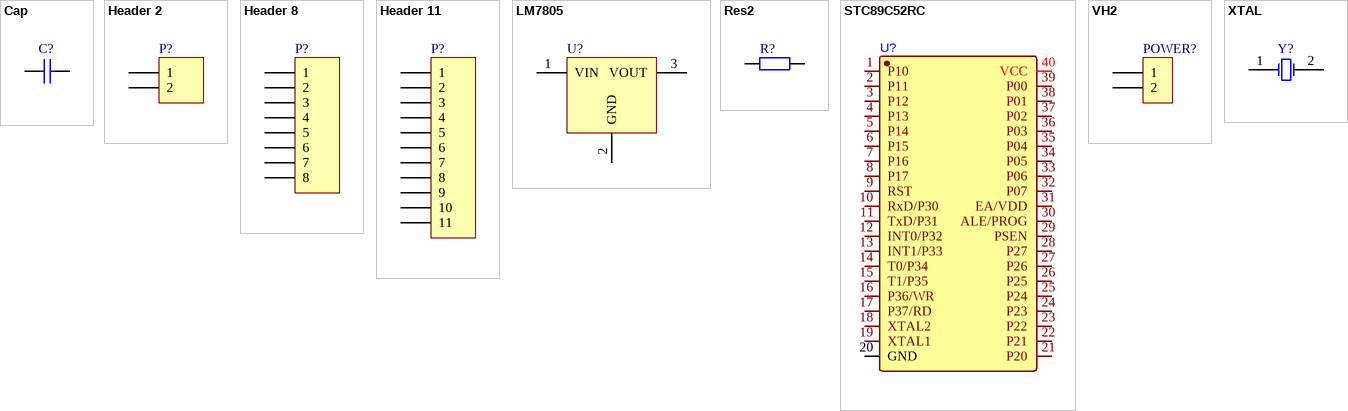
[diagram p0: symbols Cap to XTAL]
# Altium schematic symbol library MISC80679-3.SCHLIB: 9 symbols
Pins are listed as number, name and electrical type; pins without a type are passive.


## Cap
designator C?
Capacitor
simulation model CAP (Capacitor)
signal-integrity model Cap
footprint CC 1.8*3.6 (pin pitch 1.8mm, diameter 3.6mm)
pins: 1, 2

## Header 2
designator P?
Header, 2-Pin
footprint HDR1X2 (Connector; Header; 2 Position)
signal-integrity model Connector
pins: 1, 2

## Header 8
designator P?
Header, 8-Pin
footprint HDR1X8 (Connector; Header; 8 Position)
signal-integrity model Connector
pins: 1, 2, 3, 4, 5, 6, 7, 8

## Header 11
designator P?
Header, 11-Pin
footprint HDR1X11 (Connector; Header; 11 Position)
signal-integrity model Connector
pins: 1, 2, 3, 4, 5, 6, 7, 8, 9, 10, 11

## LM7805
designator U?
footprint TO220A (220, 3-pin transistor)
footprint TO252 (252 transistor)
pins: 1 VIN, 2 GND, 3 VOUT

## Res2
designator R?
Resistor
footprint AXIAL-0.4 (Axial Device, Thru-Hole; 2 Leads; 0.4 in Pin Spacing)
simulation model RESISTOR (Resistor)
signal-integrity model Res
pins: 1, 2

## STC89C52RC
designator U?
footprint STC89C52RC
pins: 1 P10, 2 P11, 3 P12, 4 P13, 5 P14, 6 P15, 7 P16, 8 P17, 9 RST, 10 RxD/P30, 11 TxD/P31, 12 INT0/P32, 13 INT1/P33, 14 T0/P34, 15 T1/P35, 16 P36/WR, 17 P37/RD, 18 XTAL2, 19 XTAL1, 20 GND, 21 P20, 22 P21, 23 P22, 24 P23, 25 P24, 26 P25, 27 P26, 28 P27, 29 PSEN, 30 ALE/PROG, 31 EA/VDD, 32 P07, 33 P06, 34 P05, 35 P04, 36 P03, 37 P02, 38 P01, 39 P00, 40 VCC

## VH2
designator POWER?
footprint VH3.96-2A
footprint VH3.96-2AW
footprint VH3.96-2AWD
pins: 1, 2

## XTAL
designator Y?
Crystal Oscillator
footprint R38 (Crystal, Thru-Hole; 2 Leads; Body 3.1 x 8.2 mm (Dia.xH))
simulation model XTAL (Spice Subcircuit)
pins: 1 OSC1, 2 OSC2